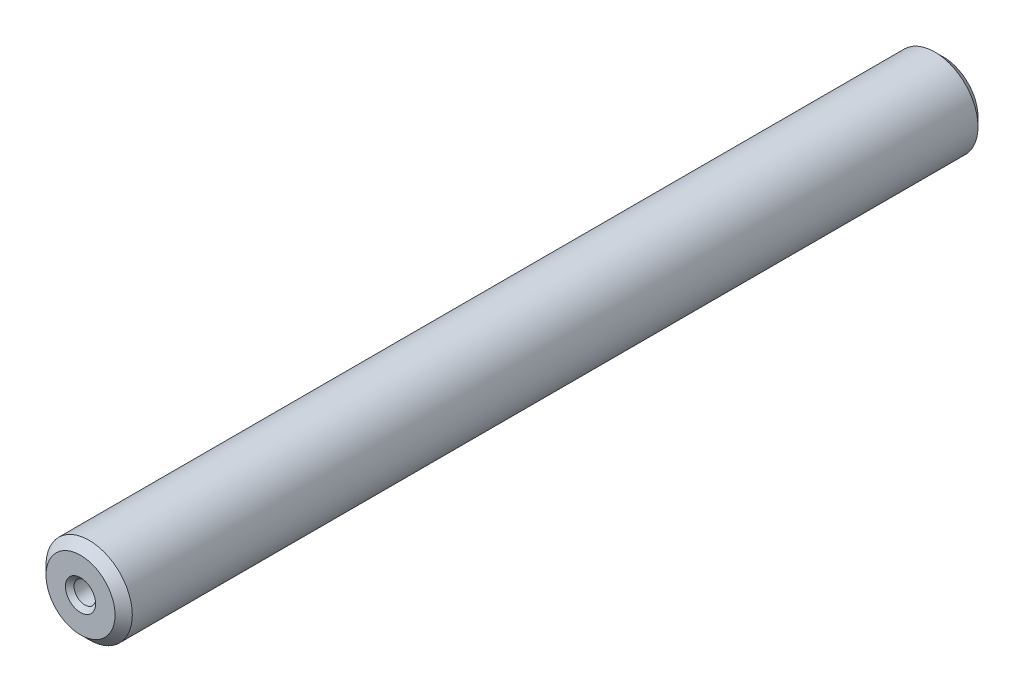
SolidWorks part; units mm, degrees
material "304"
ref_plane "Front Plane" through (0, 0, 0) normal (0, 0, 1) x (1, 0, 0)
ref_plane "Top Plane" through (0, 0, 0) normal (0, 1, 0) x (1, 0, 0)
ref_plane "Right Plane" through (0, 0, 0) normal (1, 0, 0) x (0, 0, -1)
sketch "Sketch1" plane through (0, 0, 0) normal (0, 0, 1) x (1, 0, 0)
  circle A0 centre (0, 0) radius 5
  dimension "D1" = 10
extrude "Boss-Extrude1" add sketch "Sketch1" along normal blind 100
hole_wizard "M3 Tapped Hole1" positions "Sketch4" profile "Sketch3" tap size "M3" standard "GB"
sketch "Sketch4" plane through (0, 0, 100) normal (0, 0, 1) x (1, 0, 0)
  point P0 (0, 0)
sketch "Sketch3" plane through (0, 0, 100) normal (1, 0, 0) x (0, -1, 0)
  line L0 (0, 0) -> (0, 7.2511)
  line L1 (0, 7.2511) -> (1.25, 6.5)
  line L2 (1.25, 6.5) -> (1.25, 0)
  line L5 (1.25, 0) -> (0, 0)
  line L10 (0, 7.2511) -> (-1.25, 6.5) construction
  line L11 (0, -6.35) -> (0, 107.95) construction
  dimension "螺纹孔钻头直径" = 2.5
  dimension "螺纹孔钻头深度" = 6.5
  dimension "导头角度" = 118
cosmetic thread "Cosmetic Thread3" parameters "D1"=5, "D2"=3
chamfer "Chamfer1" distance 1 angle 45 2 edges at (5, 0, 0) (5, 0, 100)
chamfer "Chamfer2" distance 0.5 angle 45 1 edges at (1.25, 0, 100)
